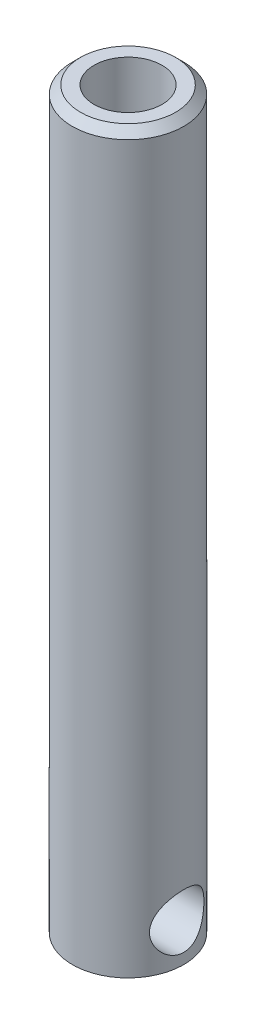
from build123d import *

# Parameters (mm, degrees)
SKETCH1_R               = 205
SKETCH1_R_2             = 125
BOSS_EXTRUDE1_DEPTH     = 2300
BOSS_EXTRUDE2_START     = 400
SKETCH2_R               = 205
BOSS_EXTRUDE2_DEPTH     = 400
CUT_EXTRUDE1_DEPTH      = 5000
CUT_EXTRUDE1_DEPTH_BACK = 4000
SKETCH3_R               = 100
CHAMFER1_SIZE           = 30


with BuildPart() as part:
    # Sketch1 → Boss-Extrude1 (new body)
    with BuildSketch(Plane(origin=(0, 0, 0), x_dir=(1, 0, 0), z_dir=(0, 1, 0))):
        with Locations(Location((0, 0, 0), (0, 0, 270))):
            Circle(SKETCH1_R)
        with Locations(Location((0, 0, 0), (0, 0, 270))):
            Circle(SKETCH1_R_2, mode=Mode.SUBTRACT)
    extrude(amount=BOSS_EXTRUDE1_DEPTH)

    # Sketch2 → Boss-Extrude2 (add)
    with BuildSketch(Plane.XZ.offset(BOSS_EXTRUDE2_START)):
        with Locations(Location((0, 0, 0), (0, 0, 270))):
            Circle(SKETCH2_R)
    extrude(amount=-BOSS_EXTRUDE2_DEPTH)

    # Sketch3 → Cut-Extrude1 (cut, two sides: drawn at the far end of the back side and taken through both)
    with BuildSketch(Plane(origin=(0, 0, 0), x_dir=(0, 0, -1), z_dir=(1, 0, 0)).offset(-CUT_EXTRUDE1_DEPTH_BACK)):
        with Locations(Location((0, -260.843725605, 0), (0, 0, 180))):
            Circle(SKETCH3_R)
    extrude(amount=CUT_EXTRUDE1_DEPTH + CUT_EXTRUDE1_DEPTH_BACK, mode=Mode.SUBTRACT)

    # Chamfer1
    chamfer1_edges = [part.edges().sort_by_distance(p)[0] for p in [
        (0, 2300, -205),
    ]]
    chamfer(chamfer1_edges, length=CHAMFER1_SIZE)


solid = part.part
